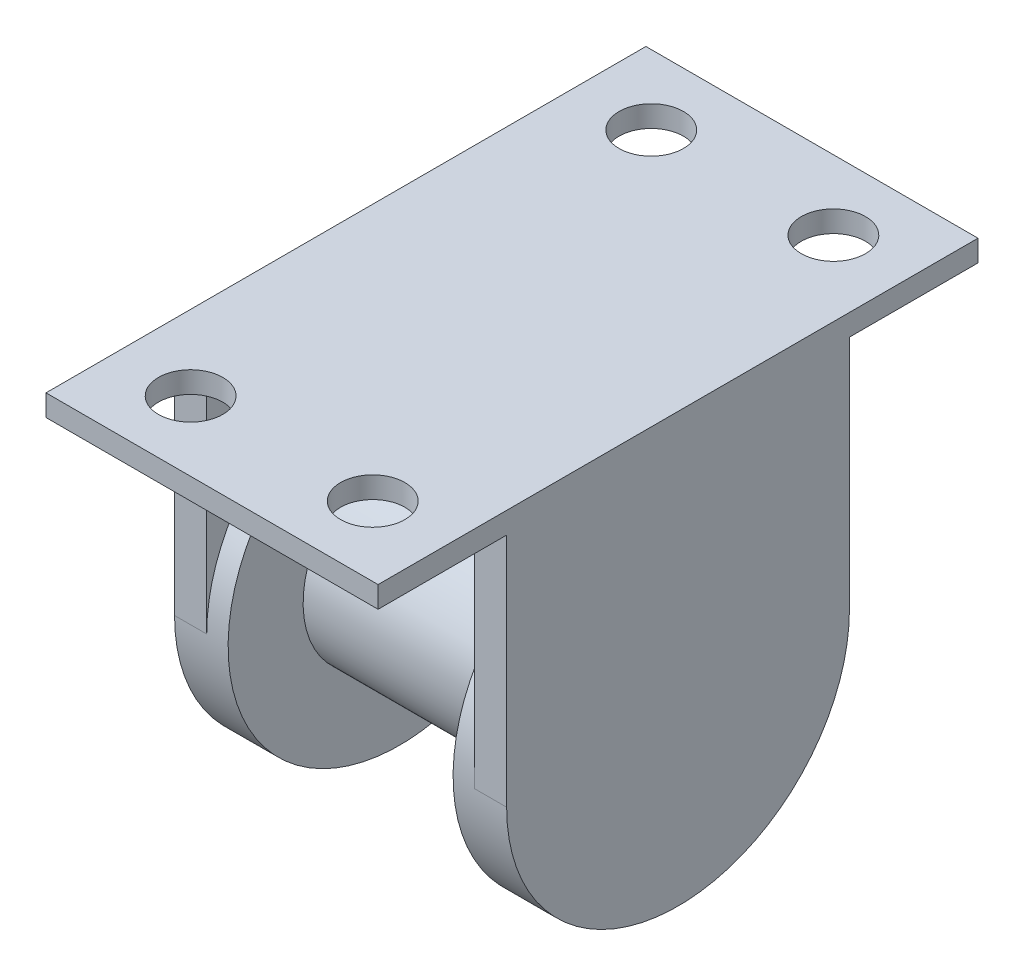
SolidWorks part; units mm, degrees
ref_plane "前视基准面" through (0, 0, 0) normal (0, 0, 1) x (1, 0, 0)
ref_plane "上视基准面" through (0, 0, 0) normal (0, 1, 0) x (1, 0, 0)
ref_plane "右视基准面" through (0, 0, 0) normal (1, 0, 0) x (0, 0, -1)
sketch "草图1" plane through (0, 0, 0) normal (0, 0, 1) x (1, 0, 0)
  line L0 (0, 18.5506) -> (0, -27.6705) construction
  line L1 (0, 16) -> (2, 16)
  line L2 (2, 16) -> (2, 9)
  line L3 (2, 9) -> (23, 9)
  line L4 (23, 9) -> (23, 16)
  line L5 (23, 16) -> (25, 16)
  line L6 (25, 16) -> (25, 0)
  line L7 (25, 0) -> (-25, 0)
  line L8 (0, 16) -> (0, 0)
  point P12 (0, 0)
  dimension "D1" = 21
  dimension "D2" = 16
  dimension "D3" = 2
  dimension "D4" = 2
  dimension "D5" = 9
revolve "旋转1" add sketch "草图1" angle 360 about L7
sketch "草图2" plane through (0, 0, 0) normal (-1, 0, 0) x (0, 0, 1)
  line L2 (-16, 0) -> (-16, 24)
  line L3 (-16, 24) -> (16, 24)
  line L4 (16, 0) -> (16, 24)
  arc A0 (-16, 0) -> (16, 0) centre (0, 0) ccw
  point P0 (0, 0)
  dimension "D1" = 24
extrude "凸台-拉伸1" add sketch "草图2" along normal blind 3
ref_plane "基准面1" through (12.5, 0, 0) normal (1, 0, 0) x (0, 0, -1)
mirror "镜向1" about plane through (12.5, 0, 0) normal (1, 0, 0) of "凸台-拉伸1"
sketch "草图4" plane through (0, 0, 0) normal (0, 0, 1) x (1, 0, 0)
  line L0 (28, 0) -> (28, 24) construction
  line L1 (-3, 24) -> (28, 24)
  line L2 (-3, 24) -> (-3, 22)
  line L3 (-3, 22) -> (28, 22)
  line L4 (28, 24) -> (28, 22)
  dimension "D1" = 2
extrude "凸台-拉伸2" add sketch "草图4" along normal mid plane 56
sketch "草图5" plane through (0, 24, 0) normal (0, 1, 0) x (1, 0, 0)
  line L0 (-3, 0) -> (28, 0) construction
  line L1 (-3, -28) -> (-3, 28) construction
  line L2 (28, -28) -> (28, 28) construction
  line L3 (12.5, 28) -> (12.5, -28) construction
  line L4 (28, 28) -> (-3, 28) construction
  line L5 (28, -28) -> (-3, -28) construction
  circle A0 centre (4, 21.5) radius 3
  circle A1 centre (4, -21.5) radius 3
  circle A2 centre (21, -21.5) radius 3
  circle A3 centre (21, 21.5) radius 3
  dimension "D1" = 6
  dimension "D2" = 43
  dimension "D3" = 17
extrude "切除-拉伸1" cut sketch "草图5" against normal up to next
